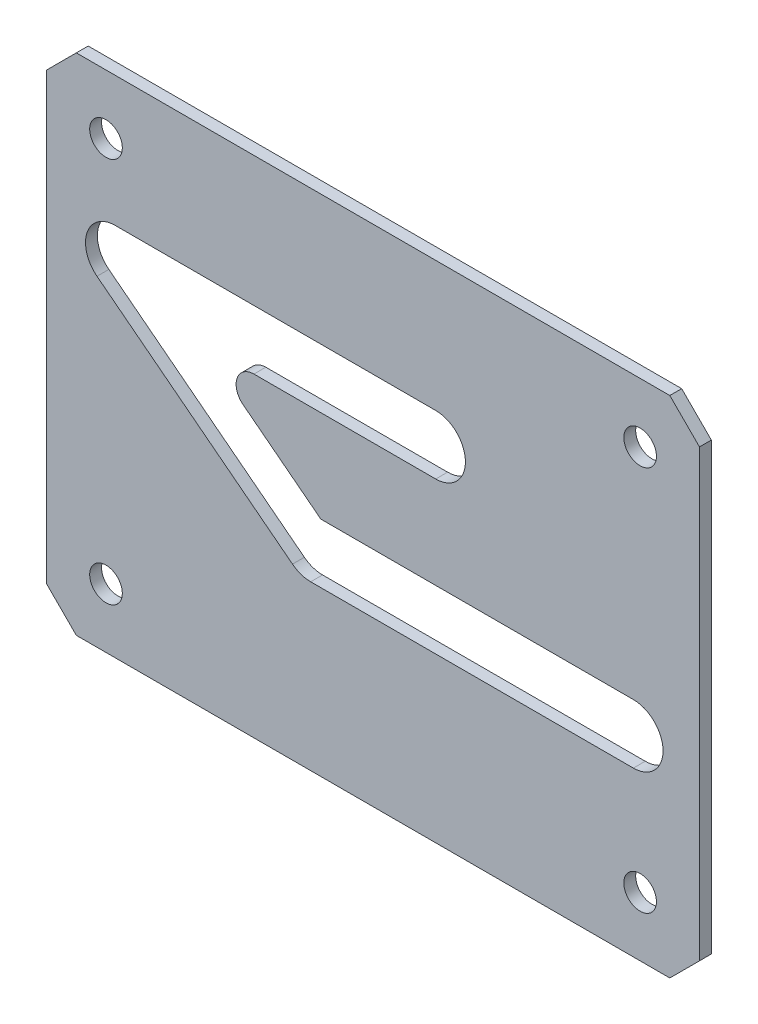
from build123d import *

# Parameters (mm, degrees)
EXTRUDE_1_DEPTH              = 1
HOLE_WIZARD_M6_1_D           = 6.6
HOLE_WIZARD_M6_1_CBORE_D     = 11
HOLE_WIZARD_M6_1_CBORE_DEPTH = 6.4
SKETCH_27_W                  = 153
SKETCH_27_H                  = 120
EXTRUDE_3_DEPTH              = 2
HOLE_WIZARD_M5_2_D           = 4.2
HOLE_WIZARD_M5_2_DEPTH       = 14
HOLE_WIZARD_M5_2_TIP         = 1.2618073
SKETCH_15_W                  = 112.889805259
SKETCH_15_H                  = 130.002769253
CUT_EXTRUDE_1_DEPTH          = 512.721848273
SKETCH_16_R                  = 10
CUT_EXTRUDE_2_DEPTH          = 2
SKETCH_18_R                  = 10
CUT_EXTRUDE_4_DEPTH          = 2
SKETCH_28_W                  = 266.209573984
SKETCH_28_H                  = 254.96875003
CUT_EXTRUDE_7_DEPTH          = 512.721848273
SKETCH_29_W                  = 20
SKETCH_29_H                  = 197
EXTRUDE_4_DEPTH              = 2
SKETCH_30_W                  = 160
SKETCH_30_H                  = 28
EXTRUDE_5_DEPTH              = 2
SKETCH_31_W                  = 160
SKETCH_31_H                  = 323
CUT_EXTRUDE_8_DEPTH          = 471.473431768
SKETCH_32_W                  = 27
SKETCH_32_H                  = 140
CUT_EXTRUDE_9_DEPTH          = 164.022237747
SKETCH_33_R                  = 10
EXTRUDE_6_DEPTH              = 2
EXTRUDE_7_DEPTH              = 2
HOLE_WIZARD_M6_2_D           = 6.6
HOLE_WIZARD_M6_2_CBORE_D     = 11
HOLE_WIZARD_M6_2_CBORE_DEPTH = 6.4
SKETCH_38_W                  = 13
SKETCH_38_H                  = 160
CUT_EXTRUDE_10_DEPTH         = 10
SKETCH_39_W                  = 50
SKETCH_39_H                  = 110.0725
EXTRUDE_8_DEPTH              = 2
SKETCH_40_W                  = 120
SKETCH_40_H                  = 49.9275
CUT_EXTRUDE_11_DEPTH         = 185.727502013
HOLE_WIZARD_5_5_5_5_1_D      = 5.5
MOVE_FACE_1_BY               = 7.5
MOVE_FACE_2_BY               = 7.5
FILLET_4_R                   = 10
SKETCH_44_OUTSIDE_W          = 214.212
SKETCH_44_OUTSIDE_H          = 169.284
SKETCH_44_OUTSIDE_W_2        = 110
SKETCH_44_OUTSIDE_H_2        = 85
CUT_EXTRUDE_12_DEPTH         = 191.47440773
CHAMFER_1_SIZE               = 5
HOLE_WIZARD_5_5_5_5_2_D      = 5.5
CUT_EXTRUDE_13_DEPTH         = 10


with BuildPart() as part:
    # Model → 凸台-拉伸1 (new, symmetric)
    with BuildSketch(Plane.XY):
        with BuildLine():
            Line((186.507023758, 241.511944981), (58.910891188, 92.809685219))
            ThreePointArc((58.910891188, 92.809685219), (57.122071441, 89.769692994), (56.5, 86.297740238))
            Line((56.5, 86.297740238), (56.5, 0))
            Line((56.5, 0), (-73.5, 0))
            ThreePointArc((-73.5, 0), (-80.571067812, 2.928932188), (-83.5, 10))
            Line((-83.5, 10), (-83.5, 335))
            Line((-83.5, 335), (59.5, 335))
            ThreePointArc((59.5, 335), (66.571067812, 337.928932188), (69.5, 345))
            Line((69.5, 345), (69.5, 435))
            Line((69.5, 435), (259.5, 435))
            ThreePointArc((259.5, 435), (266.571067812, 432.071067812), (269.5, 425))
            Line((269.5, 425), (269.5, 255))
            ThreePointArc((269.5, 255), (266.571067812, 247.928932188), (259.5, 245))
            Line((259.5, 245), (194.09613257, 245))
            ThreePointArc((194.09613257, 245), (189.91997703, 244.086238215), (186.507023758, 241.511944981))
        make_face()
    extrude(amount=EXTRUDE_1_DEPTH, both=True)

    # M6 六角凹头螺钉的柱形沉头孔1 (through all)
    with Locations(Plane(origin=(0, 0, -1), x_dir=(-1, 0, 0), z_dir=(0, 0, -1))):
        with Locations((16.5, 157), (-9.5, 235), (-9.5, 157), (16.5, 235)):
            CounterBoreHole(HOLE_WIZARD_M6_1_D / 2, HOLE_WIZARD_M6_1_CBORE_D / 2, HOLE_WIZARD_M6_1_CBORE_DEPTH)

    # 草图27 → 凸台-拉伸3 (add)
    with BuildSketch(Plane.XY.offset(1)):
        with Locations((-7, 375)):
            Rectangle(SKETCH_27_W, SKETCH_27_H)
    extrude(amount=-EXTRUDE_3_DEPTH)

    # M5 螺纹孔2
    with Locations(Plane.XY.offset(1)):
        with Locations((-60.5, 390), (27.5, 405), (47.5, 265), (-32.5, 270)):
            Hole(HOLE_WIZARD_M5_2_D / 2, depth=HOLE_WIZARD_M5_2_DEPTH)
            with Locations((0, 0, -(HOLE_WIZARD_M5_2_DEPTH + HOLE_WIZARD_M5_2_TIP / 2))):  # 118° drill point
                Cone(0, HOLE_WIZARD_M5_2_D / 2, HOLE_WIZARD_M5_2_TIP, mode=Mode.SUBTRACT)

    # 草图15 → 切除-拉伸1 (cut, through all)
    with BuildSketch(Plane.XY.offset(1)):
        with Locations((112.94490263, 131.998615374)):
            Rectangle(SKETCH_15_W, SKETCH_15_H)
    extrude(amount=-CUT_EXTRUDE_1_DEPTH, mode=Mode.SUBTRACT)

    # 草图16 → 切除-拉伸2 (cut)
    with BuildSketch(Plane.XY.offset(1)):
        with Locations((-13.5, 25)):
            Circle(SKETCH_16_R)
    cut_extrude_2 = extrude(amount=-CUT_EXTRUDE_2_DEPTH, mode=Mode.SUBTRACT)

    # 草图18 → 切除-拉伸4 (cut)
    with BuildSketch(Plane.XY.offset(1)):
        with Locations((244.5, 340)):
            Circle(SKETCH_18_R)
    extrude(amount=-CUT_EXTRUDE_4_DEPTH, mode=Mode.SUBTRACT)

    # 草图28 → 切除-拉伸7 (cut, through all)
    with BuildSketch(Plane.XY.offset(1)):
        with Locations((209.604786992, 307.515624985)):
            Rectangle(SKETCH_28_W, SKETCH_28_H)
    extrude(amount=-CUT_EXTRUDE_7_DEPTH, mode=Mode.SUBTRACT)

    # 草图29 → 凸台-拉伸4 (add)
    with BuildSketch(Plane.XY.offset(1)):
        with Locations((66.5, 98.5)):
            Rectangle(SKETCH_29_W, SKETCH_29_H)
    extrude(amount=-EXTRUDE_4_DEPTH)

    # 草图30 → 凸台-拉伸5 (add)
    with BuildSketch(Plane.XY.offset(1)):
        with Locations((-3.5, 449)):
            Rectangle(SKETCH_30_W, SKETCH_30_H)
    extrude(amount=-EXTRUDE_5_DEPTH)

    # 镜向1: 切除-拉伸2 across plane
    add(cut_extrude_2.mirror(Plane.ZX.offset(231.5)), mode=Mode.SUBTRACT)

    # 草图31 → 切除-拉伸8 (cut, through all)
    with BuildSketch(Plane.XY.offset(1)):
        with Locations((-3.5, 301.5)):
            Rectangle(SKETCH_31_W, SKETCH_31_H)
    extrude(amount=-CUT_EXTRUDE_8_DEPTH, mode=Mode.SUBTRACT)

    # 草图32 → 切除-拉伸9 (cut, through all)
    with BuildSketch(Plane.XY.offset(1)):
        with Locations((63, 70)):
            Rectangle(SKETCH_32_W, SKETCH_32_H)
    extrude(amount=-CUT_EXTRUDE_9_DEPTH, mode=Mode.SUBTRACT)

    # 草图33 → 凸台-拉伸6 (add)
    with BuildSketch(Plane.XY.offset(1)):
        with Locations((-13.5, 25)):
            Circle(SKETCH_33_R)
    extrude(amount=-EXTRUDE_6_DEPTH)

    # 草图37 → 凸台-拉伸7 (add)
    with BuildSketch(Plane.XY.offset(1)):
        with BuildLine():
            Line((49.5, 0), (-73.5, 0))
            ThreePointArc((-73.5, 0), (-80.571067812, 2.928932188), (-83.5, 10))
            Line((-83.5, 10), (-83.5, -20))
            Line((-83.5, -20), (49.5, -20))
            Line((49.5, -20), (49.5, 0))
        make_face()
    extrude(amount=-EXTRUDE_7_DEPTH)

    # M6 六角凹头螺钉的柱形沉头孔2 (through all)
    with Locations(Plane.XY.offset(1)):
        with Locations((-40.5, -10), (-40.5, 15), (19.5, 15), (19.5, -10)):
            CounterBoreHole(HOLE_WIZARD_M6_2_D / 2, HOLE_WIZARD_M6_2_CBORE_D / 2, HOLE_WIZARD_M6_2_CBORE_DEPTH)

    # 草图38 → 切除-拉伸10 (cut)
    with BuildSketch(Plane.XY.offset(1)):
        with Locations((-77, 60)):
            Rectangle(SKETCH_38_W, SKETCH_38_H)
    extrude(amount=-CUT_EXTRUDE_10_DEPTH, mode=Mode.SUBTRACT)

    # 草图39 → 凸台-拉伸8 (add)
    with BuildSketch(Plane.XY.offset(1)):
        with Locations((-95.5, 84.96375)):
            Rectangle(SKETCH_39_W, SKETCH_39_H)
    extrude(amount=-EXTRUDE_8_DEPTH)

    # 草图40 → 切除-拉伸11 (cut, through all)
    with BuildSketch(Plane(origin=(0, 0, -1), x_dir=(-1, 0, 0), z_dir=(0, 0, -1))):
        with Locations((10.5, 4.96375)):
            Rectangle(SKETCH_40_W, SKETCH_40_H)
    extrude(amount=-CUT_EXTRUDE_11_DEPTH, mode=Mode.SUBTRACT)

    # Ø5.5 (5.5) 直径孔1 (through all)
    with Locations(Plane.XY.offset(1)):
        with Locations((-87.5, 57.4275), (-112.5, 57.4275), (-112.5, 117.4275), (-87.5, 117.4275)):
            Hole(HOLE_WIZARD_5_5_5_5_1_D / 2)

    # Move Face 1: a face moved outward by 7.5
    extrude(part.faces().sort_by_distance((-35.5, 29.9275, 0))[0], amount=MOVE_FACE_1_BY, dir=(0, -1, 0))

    # Move Face 2: a face moved outward by 7.5
    extrude(part.faces().sort_by_distance((-35.5, 140, 0))[0], amount=MOVE_FACE_2_BY, dir=(0, 1, 0))

    # 圆角4
    fillet_4_edges = [part.edges().sort_by_distance(p)[0] for p in [
        (49.5, 147.5, 0),
        (-120.5, 147.5, 0),
        (-120.5, 22.4275, 0),
        (49.5, 22.4275, 0),
    ]]
    fillet(fillet_4_edges, radius=FILLET_4_R)

    # 草图44 outside → 切除-拉伸12 (cut, through all)
    with BuildSketch(Plane.XY.offset(1)):
        with Locations((-35.5, 84.964)):
            Rectangle(SKETCH_44_OUTSIDE_W, SKETCH_44_OUTSIDE_H)
        with Locations((-10.5, 87.4275)):
            Rectangle(SKETCH_44_OUTSIDE_W_2, SKETCH_44_OUTSIDE_H_2, mode=Mode.SUBTRACT)
    extrude(amount=-CUT_EXTRUDE_12_DEPTH, mode=Mode.SUBTRACT)

    # 倒角1
    chamfer_1_edges = [part.edges().sort_by_distance(p)[0] for p in [
        (-65.5, 129.9275, 0),
        (44.5, 129.9275, 0),
        (44.5, 44.9275, 0),
        (-65.5, 44.9275, 0),
    ]]
    chamfer(chamfer_1_edges, length=CHAMFER_1_SIZE)

    # Ø5.5 (5.5) 直径孔2 (through all)
    with Locations(Plane.XY.offset(1)):
        with Locations((34.5, 54.9275), (34.5, 119.9275), (-55.5, 119.9275), (-55.5, 54.9275)):
            Hole(HOLE_WIZARD_5_5_5_5_2_D / 2)

    # 草图45 → 切除-拉伸13 (cut)
    with BuildSketch(Plane.XY.offset(1)):
        with BuildLine():
            Line((33.36, 72.488602629), (-21.012598119, 72.488602629))
            ThreePointArc((-21.012598119, 72.488602629), (-22.631292343, 72.757870233), (-24.075641802, 73.536671027))
            Line((-24.075641802, 73.536671027), (-57.018167055, 99.06960126))
            ThreePointArc((-57.018167055, 99.06960126), (-58.685855768, 104.640227087), (-53.955123371, 108.021532863))
            Line((-53.955123371, 108.021532863), (0.06, 108.021532863))
            ThreePointArc((0.06, 108.021532863), (5.06, 103.021532863), (0.06, 98.021532863))
            Line((0.06, 98.021532863), (-30.574636438, 98.021532863))
            ThreePointArc((-30.574636438, 98.021532863), (-33.413075876, 95.992749398), (-32.412462648, 92.650373901))
            Line((-32.412462648, 92.650373901), (-19.301769764, 82.488602629))
            Line((-19.301769764, 82.488602629), (33.36, 82.488602629))
            ThreePointArc((33.36, 82.488602629), (38.36, 77.488602629), (33.36, 72.488602629))
        make_face()
    extrude(amount=-CUT_EXTRUDE_13_DEPTH, mode=Mode.SUBTRACT)


solid = part.part
